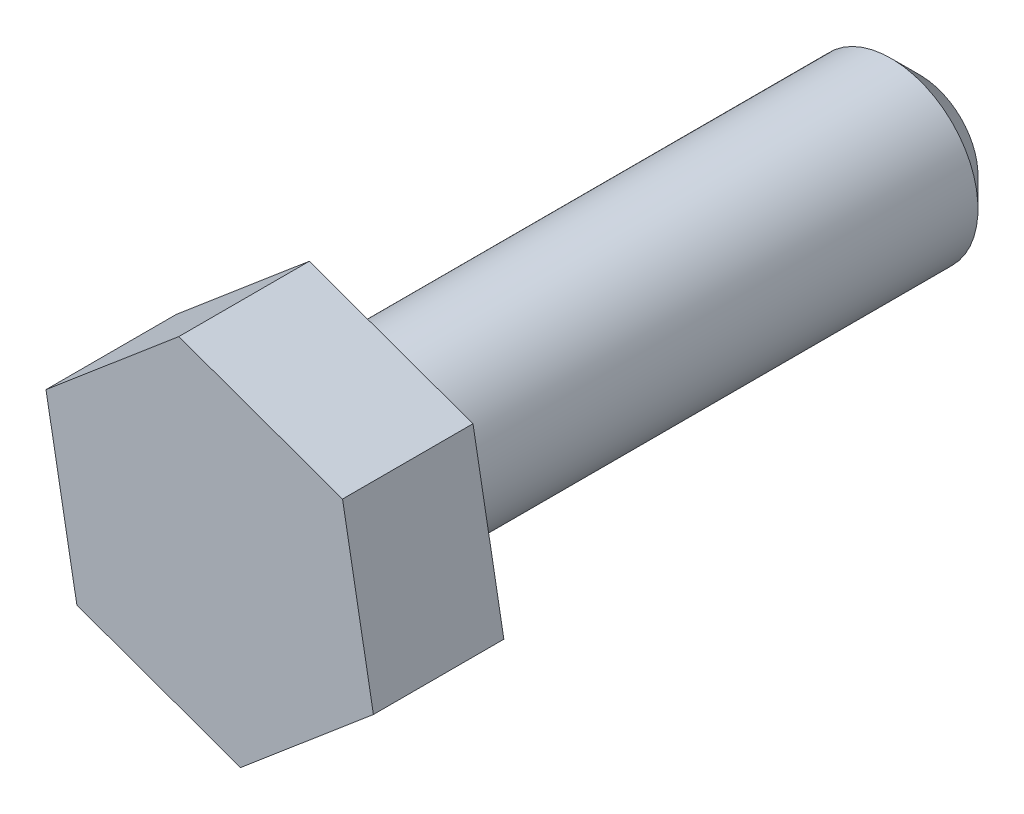
from build123d import *

# Parameters (mm, degrees)
SKETCH1_R           = 6
BOSS_EXTRUDE1_DEPTH = 4.5
SKETCH2_OUTSIDE_W   = 17.512
SKETCH2_OUTSIDE_H   = 17.512
CUT_EXTRUDE1_DEPTH  = 4.5
SKETCH3_R           = 3
BOSS_EXTRUDE2_DEPTH = 20
CHAMFER2_SIZE       = 1


with BuildPart() as part:
    # Sketch1 → Boss-Extrude1 (new body)
    with BuildSketch(Plane.XY):
        Circle(SKETCH1_R)
    extrude(amount=BOSS_EXTRUDE1_DEPTH)

    # Sketch2 outside → Cut-Extrude1 (cut)
    with BuildSketch(Plane(origin=(0, 0, 0), x_dir=(-1, 0, 0), z_dir=(0, 0, -1))):
        Rectangle(SKETCH2_OUTSIDE_W, SKETCH2_OUTSIDE_H)
        Polygon((4.581142128, -3.874678929), (5.646141448, 2.030045997), (1.06499932, 5.904724926), (-4.581142128, 3.874678929), (-5.646141448, -2.030045997), (-1.06499932, -5.904724926), align=None, mode=Mode.SUBTRACT)
    extrude(amount=-CUT_EXTRUDE1_DEPTH, mode=Mode.SUBTRACT)

    # Sketch3 → Boss-Extrude2 (add)
    with BuildSketch(Plane(origin=(0, 0, 0), x_dir=(-1, 0, 0), z_dir=(0, 0, -1))):
        Circle(SKETCH3_R)
    extrude(amount=BOSS_EXTRUDE2_DEPTH)

    # Chamfer2
    chamfer2_edges = [part.edges().sort_by_distance(p)[0] for p in [
        (3, 0, -20),
    ]]
    chamfer(chamfer2_edges, length=CHAMFER2_SIZE)


solid = part.part
